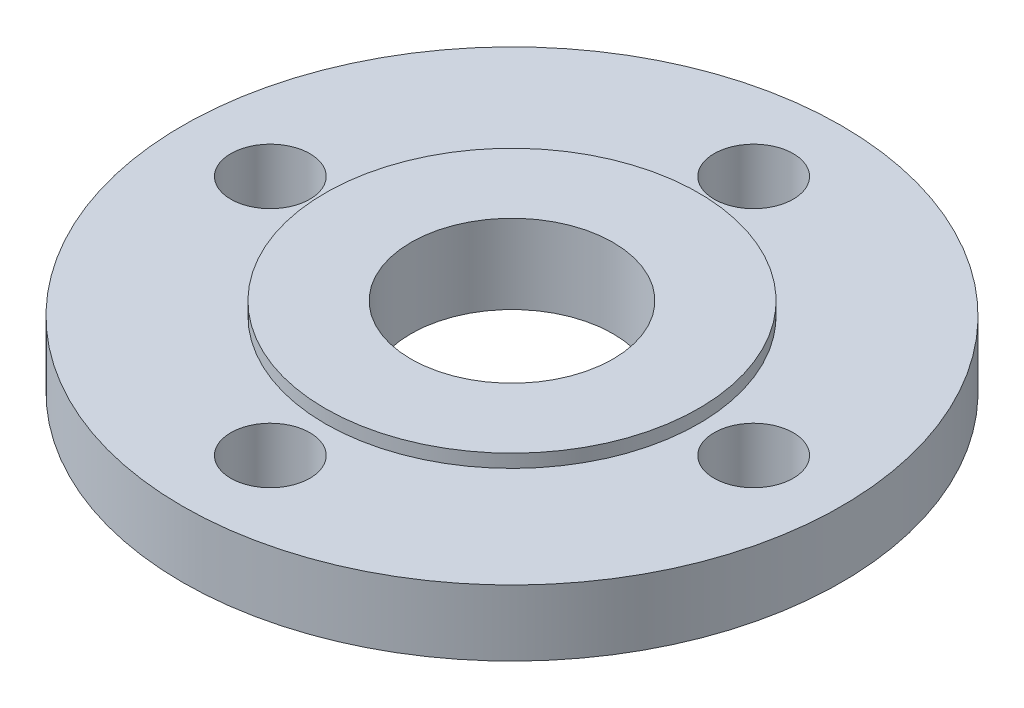
from build123d import *

# Parameters (mm, degrees)
SKETCH_1_R      = 75
SKETCH_1_R_2    = 9
SKETCH_1_R_3    = 23
EXTRUDE_1_DEPTH = 15
SKETCH_2_R      = 42.5
SKETCH_2_R_2    = 23
EXTRUDE_2_DEPTH = 3


with BuildPart() as part:
    # 草图1 → 凸台-拉伸1 (new body)
    with BuildSketch(Plane(origin=(0, 0, 0), x_dir=(1, 0, 0), z_dir=(0, 1, 0))):
        with Locations(Location((0, 0, 0), (0, 0, 270))):
            Circle(SKETCH_1_R)
        with Locations(Location((0, 55, 0), (0, 0, 270))):
            Circle(SKETCH_1_R_2, mode=Mode.SUBTRACT)
        with Locations(Location((55, 0, 0), (0, 0, 270))):
            Circle(SKETCH_1_R_2, mode=Mode.SUBTRACT)
        with Locations(Location((0, -55, 0), (0, 0, 270))):
            Circle(SKETCH_1_R_2, mode=Mode.SUBTRACT)
        with Locations(Location((-55, 0, 0), (0, 0, 270))):
            Circle(SKETCH_1_R_2, mode=Mode.SUBTRACT)
        with Locations(Location((0, 0, 0), (0, 0, 270))):
            Circle(SKETCH_1_R_3, mode=Mode.SUBTRACT)
    extrude(amount=EXTRUDE_1_DEPTH)

    # 草图2 → 凸台-拉伸2 (add)
    with BuildSketch(Plane(origin=(0, 15, 0), x_dir=(1, 0, 0), z_dir=(0, 1, 0))):
        with Locations(Location((0, 0, 0), (0, 0, 270))):
            Circle(SKETCH_2_R)
        with Locations(Location((0, 0, 0), (0, 0, 270))):
            Circle(SKETCH_2_R_2, mode=Mode.SUBTRACT)
    extrude(amount=EXTRUDE_2_DEPTH)


solid = part.part
